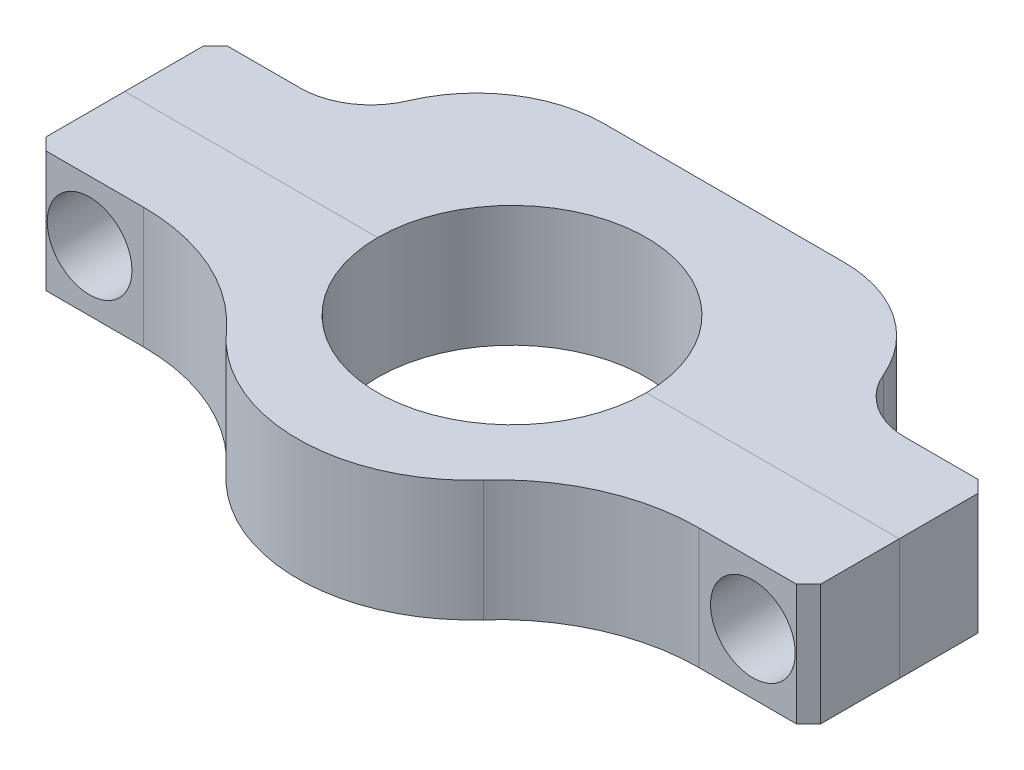
from build123d import *

# Parameters (mm, degrees)
BOSS_EXTRUDE1_DEPTH = 10
CHAMFER1_SIZE       = 1
CUT_EXTRUDE1_START  = 4.754218
SKETCH3_R           = 3.5
CUT_EXTRUDE1_DEPTH  = 20
SKETCH7_R           = 11.1
CUT_EXTRUDE2_DEPTH  = 20


with BuildPart() as part:
    # Sketch1 → Boss-Extrude1 (new body)
    with BuildSketch(Plane(origin=(0, 0, 0), x_dir=(1, 0, 0), z_dir=(0, 1, 0))):
        with BuildLine():
            Line((9.923855052, 12.745782203), (-9.923855052, 12.745782203))
            ThreePointArc((-9.923855052, 12.745782203), (-15.7379694, 10.992816749), (-19.614159094, 6.318207995))
            ThreePointArc((-19.614159094, 6.318207995), (-21.768533293, 3.720074961), (-25, 2.745782203))
            Line((-25, 2.745782203), (-32, 2.745782203))
            Line((-32, 2.745782203), (-32, -12.254217797))
            Line((-32, -12.254217797), (-22.930291583, -12.254217797))
            ThreePointArc((-22.930291583, -12.254217797), (-16.191557905, -13.687244076), (-10.619046633, -17.738319737))
            ThreePointArc((-10.619046633, -17.738319737), (0, -22.468623982), (10.619046633, -17.738319737))
            ThreePointArc((10.619046633, -17.738319737), (16.191557905, -13.687244076), (22.930291583, -12.254217797))
            Line((22.930291583, -12.254217797), (32, -12.254217797))
            Line((32, -12.254217797), (32, 2.745782203))
            Line((32, 2.745782203), (25, 2.745782203))
            ThreePointArc((25, 2.745782203), (21.768533293, 3.720074961), (19.614159094, 6.318207995))
            ThreePointArc((19.614159094, 6.318207995), (15.7379694, 10.992816749), (9.923855052, 12.745782203))
        make_face()
    extrude(amount=BOSS_EXTRUDE1_DEPTH)

    # Chamfer1
    chamfer1_edges = [part.edges().sort_by_distance(p)[0] for p in [
        (32, 5, -2.745782203),
        (32, 5, 12.254217797),
        (-32, 5, 12.254217797),
        (-32, 5, -2.745782203),
    ]]
    chamfer(chamfer1_edges, length=CHAMFER1_SIZE)

    # Sketch3 → Cut-Extrude1 (cut)
    with BuildSketch(Plane.XY.offset(CUT_EXTRUDE1_START)):
        with Locations((27.40080015, 5)):
            Circle(SKETCH3_R)
        with Locations(Location((-27.40080015, 5, 0), (0, 0, 180))):
            Circle(SKETCH3_R)
    extrude(amount=CUT_EXTRUDE1_DEPTH, mode=Mode.SUBTRACT)

    # Sketch7 → Cut-Extrude2 (cut)
    with BuildSketch(Plane(origin=(0, 10, 0), x_dir=(1, 0, 0), z_dir=(0, 1, 0))):
        with Locations(Location((0, -4.754217797, 0), (0, 0, 180))):
            Circle(SKETCH7_R)
    extrude(amount=-CUT_EXTRUDE2_DEPTH, mode=Mode.SUBTRACT)


solid = part.part
